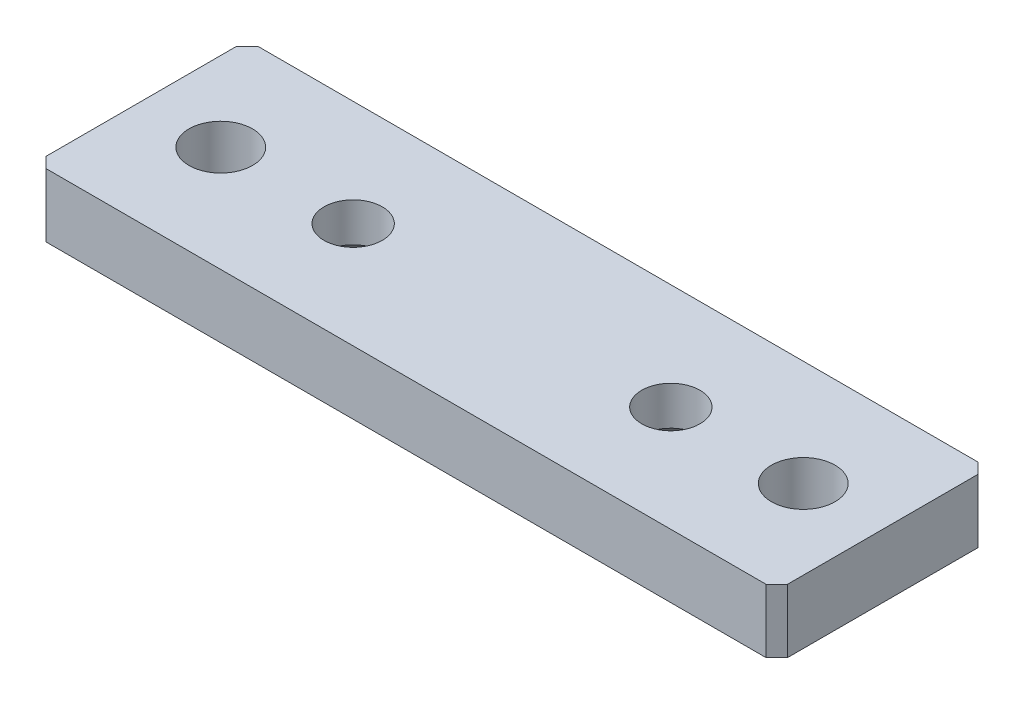
from build123d import *

# Parameters (mm, degrees)
SKETCH5_W                                         = 140
SKETCH5_H                                         = 40
BOSS_EXTRUDE1_DEPTH                               = 12
M10_CLEARANCE_HOLE1_D                             = 12
M10_CLEARANCE_HOLE1_DEPTH                         = 53
M10_CLEARANCE_HOLE1_TIP                           = 3.605163714
HOLE_SIZE_BASED_HEX_SOCKET_COUNTERSUN_D           = 11
HOLE_SIZE_BASED_HEX_SOCKET_COUNTERSUN_DEPTH       = 53
HOLE_SIZE_BASED_HEX_SOCKET_COUNTERSUN_CSINK_D     = 20.3
HOLE_SIZE_BASED_HEX_SOCKET_COUNTERSUN_CSINK_ANGLE = 90
HOLE_SIZE_BASED_HEX_SOCKET_COUNTERSUN_TIP         = 3.304733405
CHAMFER1_SIZE                                     = 2


with BuildPart() as part:
    # Sketch5 → Boss-Extrude1 (new body)
    with BuildSketch(Plane(origin=(0, 0, 0), x_dir=(1, 0, 0), z_dir=(0, 1, 0))):
        Rectangle(SKETCH5_W, SKETCH5_H)
    extrude(amount=BOSS_EXTRUDE1_DEPTH)

    # M10 Clearance Hole1
    with Locations(Plane(origin=(0, 12, 0), x_dir=(1, 0, 0), z_dir=(0, 1, 0))):
        with Locations((-55, 0), (55, 0)):
            Hole(M10_CLEARANCE_HOLE1_D / 2, depth=M10_CLEARANCE_HOLE1_DEPTH)
            with Locations((0, 0, -(M10_CLEARANCE_HOLE1_DEPTH + M10_CLEARANCE_HOLE1_TIP / 2))):  # 118° drill point
                Cone(0, M10_CLEARANCE_HOLE1_D / 2, M10_CLEARANCE_HOLE1_TIP, mode=Mode.SUBTRACT)

    # Hole size (%-based) hex socket countersunk screw type2
    with Locations(Plane(origin=(0, 0, 0), x_dir=(-1, 0, 0), z_dir=(0, -1, 0))):
        with Locations((-30, 0), (30, 0)):
            CounterSinkHole(HOLE_SIZE_BASED_HEX_SOCKET_COUNTERSUN_D / 2, HOLE_SIZE_BASED_HEX_SOCKET_COUNTERSUN_CSINK_D / 2, depth=HOLE_SIZE_BASED_HEX_SOCKET_COUNTERSUN_DEPTH, counter_sink_angle=HOLE_SIZE_BASED_HEX_SOCKET_COUNTERSUN_CSINK_ANGLE)
            with Locations((0, 0, -(HOLE_SIZE_BASED_HEX_SOCKET_COUNTERSUN_DEPTH + HOLE_SIZE_BASED_HEX_SOCKET_COUNTERSUN_TIP / 2))):  # 118° drill point
                Cone(0, HOLE_SIZE_BASED_HEX_SOCKET_COUNTERSUN_D / 2, HOLE_SIZE_BASED_HEX_SOCKET_COUNTERSUN_TIP, mode=Mode.SUBTRACT)

    # Chamfer1
    chamfer1_edges = [part.edges().sort_by_distance(p)[0] for p in [
        (70, 6, 20),
        (-70, 6, 20),
        (-70, 6, -20),
        (70, 6, -20),
    ]]
    chamfer(chamfer1_edges, length=CHAMFER1_SIZE)


solid = part.part
